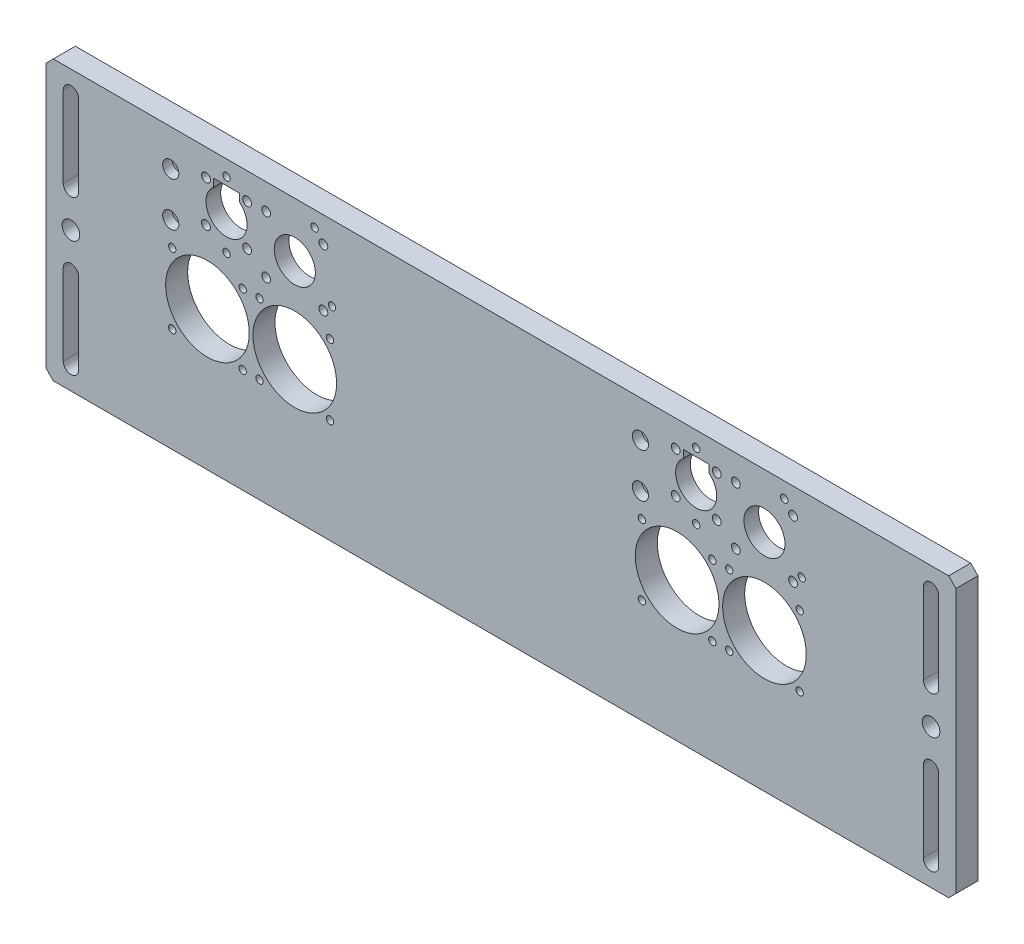
from build123d import *

# Parameters (mm, degrees)
SKETCH1_W                                           = 620
SKETCH1_H                                           = 190
BOSS_EXTRUDE1_DEPTH                                 = 15
CUT_EXTRUDE1_DEPTH                                  = 567.364076537
CUT_EXTRUDE1_DEPTH_BACK                             = 567.364076537
SKETCH2_R                                           = 6
CUT_EXTRUDE2_DEPTH                                  = 567.364076537
LPATTERN1_COUNT                                     = 2
LPATTERN1_PITCH                                     = 586
CHAMFER1_SIZE                                       = 5
SKETCH6_W                                           = 100
SKETCH6_H                                           = 56
CUT_EXTRUDE3_DEPTH                                  = 5
FILLET1_R                                           = 2.5
SKETCH7_R                                           = 14
SKETCH7_R_2                                         = 3
CUT_EXTRUDE4_DEPTH                                  = 567.25371274
M6_TAPPED_HOLE1_D                                   = 5
M6_TAPPED_HOLE2_D                                   = 5
SKETCH12_R                                          = 28.5
CUT_EXTRUDE5_DEPTH                                  = 567.364076537
SKETCH13_R                                          = 28.5
CUT_EXTRUDE6_DEPTH                                  = 567.364076537
M6_TAPPED_HOLE3_D                                   = 5
LPATTERN5_COUNT                                     = 2
LPATTERN5_PITCH                                     = 320
FILLET1_OF_LPATTERN5_R                              = 2.5
CBORE_FOR_M6_HEX_SOCKET_HEAD_CAP_SCREW1_D           = 6.6
CBORE_FOR_M6_HEX_SOCKET_HEAD_CAP_SCREW1_CBORE_D     = 11
CBORE_FOR_M6_HEX_SOCKET_HEAD_CAP_SCREW1_CBORE_DEPTH = 6.4


with BuildPart() as part:
    # Sketch1 → Boss-Extrude1 (new body)
    with BuildSketch(Plane.XY):
        with Locations((247.327777778, 4.644444444)):
            Rectangle(SKETCH1_W, SKETCH1_H)
    extrude(amount=BOSS_EXTRUDE1_DEPTH)

    # Sketch2 → Cut-Extrude1 (cut, two sides: drawn at the far end of the back side and taken through both)
    with BuildSketch(Plane.XY.offset(15).offset(-CUT_EXTRUDE1_DEPTH_BACK)):
        with Locations((-45.672222222, 4.644444444)):
            Circle(SKETCH2_R)
        with Locations((540.327777778, 4.644444444)):
            Circle(SKETCH2_R)
    extrude(amount=CUT_EXTRUDE1_DEPTH + CUT_EXTRUDE1_DEPTH_BACK, mode=Mode.SUBTRACT)

    # Sketch5 → Cut-Extrude2 (cut, symmetric)
    with BuildSketch(Plane.XY.offset(15)):
        with BuildLine():
            Line((-40.422222222, 84.644444444), (-40.422222222, 29.644444444))
            ThreePointArc((-40.422222222, 29.644444444), (-45.672222222, 24.394444444), (-50.922222222, 29.644444444))
            Line((-50.922222222, 29.644444444), (-50.922222222, 84.644444444))
            ThreePointArc((-50.922222222, 84.644444444), (-45.672222222, 89.894444444), (-40.422222222, 84.644444444))
        make_face()
        with BuildLine():
            Line((-40.422222222, -20.355555556), (-40.422222222, -75.355555556))
            ThreePointArc((-40.422222222, -75.355555556), (-45.672222222, -80.605555556), (-50.922222222, -75.355555556))
            Line((-50.922222222, -75.355555556), (-50.922222222, -20.355555556))
            ThreePointArc((-50.922222222, -20.355555556), (-45.672222222, -15.105555556), (-40.422222222, -20.355555556))
        make_face()
    cut_extrude2 = extrude(amount=CUT_EXTRUDE2_DEPTH, both=True, mode=Mode.SUBTRACT)

    # LPattern1: Cut-Extrude2 ×2
    with Locations(*[(i * LPATTERN1_PITCH, 0, 0) for i in range(1, LPATTERN1_COUNT)]):
        add(cut_extrude2, mode=Mode.SUBTRACT)

    # Chamfer1
    chamfer1_edges = [part.edges().sort_by_distance(p)[0] for p in [
        (-62.672222222, 99.644444444, 7.5),
        (557.327777778, 99.644444444, 7.5),
        (557.327777778, -90.355555556, 7.5),
        (-62.672222222, -90.355555556, 7.5),
    ]]
    chamfer(chamfer1_edges, length=CHAMFER1_SIZE)

    # Sketch6 → Cut-Extrude3 (cut)
    with BuildSketch(Plane(origin=(0, 0, 0), x_dir=(-1, 0, 0), z_dir=(0, 0, -1))):
        with Locations((-87.327777778, 66.644444444)):
            Rectangle(SKETCH6_W, SKETCH6_H)
    cut_extrude3 = extrude(amount=-CUT_EXTRUDE3_DEPTH, mode=Mode.SUBTRACT)

    # Fillet1
    fillet1_edges = [part.edges().sort_by_distance(p)[0] for p in [
        (137.327777778, 38.644444444, 2.5),
        (137.327777778, 94.644444444, 2.5),
        (37.327777778, 94.644444444, 2.5),
        (37.327777778, 38.644444444, 2.5),
    ]]
    fillet(fillet1_edges, radius=FILLET1_R)

    # Sketch7 → Cut-Extrude4 (cut, through all)
    with BuildSketch(Plane(origin=(0, 0, 5), x_dir=(-1, 0, 0), z_dir=(0, 0, -1))):
        with Locations((-106.826165278, 62.645244444)):
            Circle(SKETCH7_R)
        with Locations((-46.34482821, 81.662196851)):
            Circle(SKETCH7_R_2)
        with Locations((-46.327677778, 53.645469444)):
            Circle(SKETCH7_R_2)
        with Locations((-74.326977778, 53.645469444)):
            Circle(SKETCH7_R_2)
        with Locations((-74.326977778, 81.644769444)):
            Circle(SKETCH7_R_2)
        with Locations((-87.326652778, 82.144756944)):
            Circle(SKETCH7_R_2)
        with Locations((-87.326652778, 43.145731944)):
            Circle(SKETCH7_R_2)
        with Locations((-126.325677778, 43.145731944)):
            Circle(SKETCH7_R_2)
        with Locations((-126.325677778, 82.144756944)):
            Circle(SKETCH7_R_2)
        with BuildLine():
            Line((-51.557722364, 83.834562358), (-69.096933191, 83.834562358))
            Line((-69.096933191, 83.834562358), (-69.096933191, 78.558140149))
            ThreePointArc((-69.096933191, 78.558140149), (-60.327327778, 53.645119444), (-51.557722364, 78.558140149))
            Line((-51.557722364, 78.558140149), (-51.557722364, 83.834562358))
        make_face()
    cut_extrude4 = extrude(amount=-CUT_EXTRUDE4_DEPTH, mode=Mode.SUBTRACT)

    # M6 Tapped Hole1 (through all)
    with Locations(Plane(origin=(0, 0, 5), x_dir=(-1, 0, 0), z_dir=(0, 0, -1))):
        with Locations((-60.327327778, 44.144444444), (-60.327327778, 89.144444444), (-132.227777778, 48.644444444), (-120.327777778, 89.144444444)):
            m6_tapped_hole1 = Hole(M6_TAPPED_HOLE1_D / 2)

    # M6 Tapped Hole2 (through all)
    with Locations(Plane.XY.offset(15)):
        with Locations((82.827777778, -19.355555556), (82.827777778, 28.644444444), (130.827777778, -19.355555556), (130.827777778, 28.644444444)):
            m6_tapped_hole2 = Hole(M6_TAPPED_HOLE2_D / 2)

    # Sketch12 → Cut-Extrude5 (cut, through all)
    with BuildSketch(Plane(origin=(0, 0, 0), x_dir=(-1, 0, 0), z_dir=(0, 0, -1))):
        with Locations((-106.827777778, 4.644444444)):
            Circle(SKETCH12_R)
    cut_extrude5 = extrude(amount=-CUT_EXTRUDE5_DEPTH, mode=Mode.SUBTRACT)

    # Sketch13 → Cut-Extrude6 (cut, symmetric)
    with BuildSketch(Plane(origin=(0, 0, 0), x_dir=(-1, 0, 0), z_dir=(0, 0, -1))):
        with Locations((-47.327777778, 4.644444444)):
            Circle(SKETCH13_R)
    cut_extrude6 = extrude(amount=CUT_EXTRUDE6_DEPTH, both=True, mode=Mode.SUBTRACT)

    # M6 Tapped Hole3 (through all)
    with Locations(Plane(origin=(0, 0, 0), x_dir=(-1, 0, 0), z_dir=(0, 0, -1))):
        with Locations((-23.327777778, -19.355555556), (-71.327777778, -19.355555556), (-23.327777778, 28.644444444), (-71.327777778, 28.644444444)):
            m6_tapped_hole3 = Hole(M6_TAPPED_HOLE3_D / 2)

    # LPattern5: Cut-Extrude3, Cut-Extrude4, M6 Tapped Hole1, M6 Tapped Hole2, Cut-Extrude5, Cut-Extrude6, M6 Tapped Hole3 ×2
    with Locations(*[(i * LPATTERN5_PITCH, 0, 0) for i in range(1, LPATTERN5_COUNT)]):
        add(cut_extrude3, mode=Mode.SUBTRACT)
        add(cut_extrude4, mode=Mode.SUBTRACT)
        add(m6_tapped_hole1, mode=Mode.SUBTRACT)
        add(m6_tapped_hole2, mode=Mode.SUBTRACT)
        add(cut_extrude5, mode=Mode.SUBTRACT)
        add(cut_extrude6, mode=Mode.SUBTRACT)
        add(m6_tapped_hole3, mode=Mode.SUBTRACT)

    # Fillet1 of LPattern5
    fillet1_of_lpattern5_edges = [part.edges().sort_by_distance(p)[0] for p in [
        (457.327777778, 38.644444444, 2.5),
        (457.327777778, 94.644444444, 2.5),
        (357.327777778, 94.644444444, 2.5),
        (357.327777778, 38.644444444, 2.5),
    ]]
    fillet(fillet1_of_lpattern5_edges, radius=FILLET1_OF_LPATTERN5_R)

    # CBORE for M6 Hex Socket Head Cap Screw1 (through all)
    with Locations(Plane.XY.offset(15)):
        with Locations((342.327777778, 44.644444444), (342.327777778, 74.644444444), (22.327777778, 44.644444444), (22.327777778, 74.644444444)):
            CounterBoreHole(CBORE_FOR_M6_HEX_SOCKET_HEAD_CAP_SCREW1_D / 2, CBORE_FOR_M6_HEX_SOCKET_HEAD_CAP_SCREW1_CBORE_D / 2, CBORE_FOR_M6_HEX_SOCKET_HEAD_CAP_SCREW1_CBORE_DEPTH)


solid = part.part
